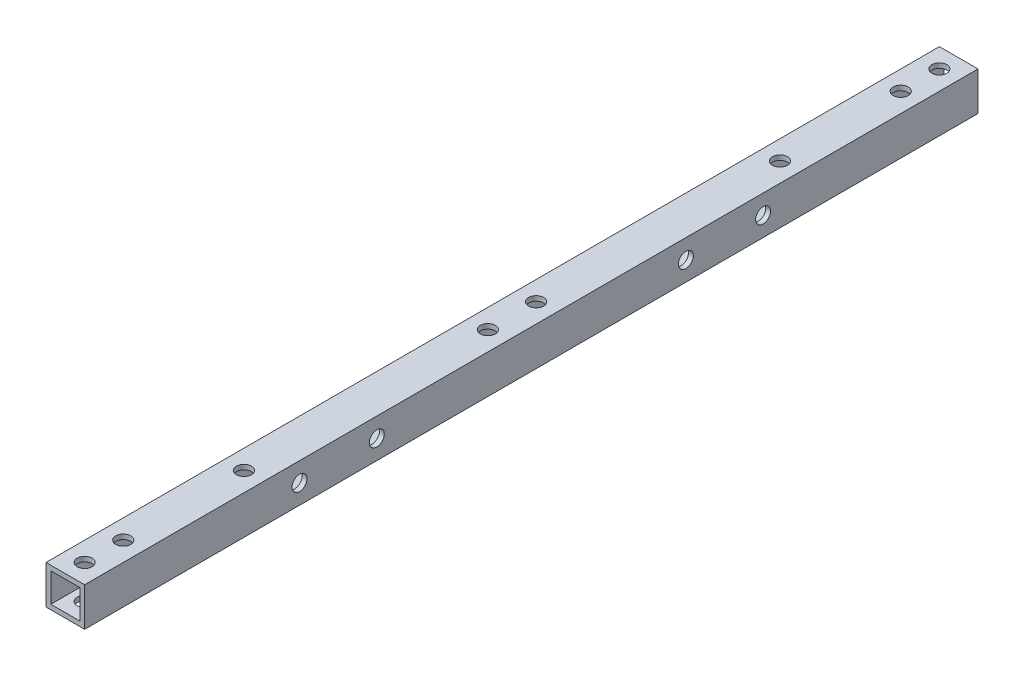
from build123d import *

# Parameters (mm, degrees)
SKETCH_1_W          = 8
SKETCH_1_H          = 8
SKETCH_1_W_2        = 6
SKETCH_1_H_2        = 6
EXTRUDE_1_DEPTH     = 185
SKETCH_2_R          = 1.55
CUT_EXTRUDE_1_DEPTH = 186.216090014
SKETCH_3_R          = 1.55
CUT_EXTRUDE_2_DEPTH = 186.216090014


with BuildPart() as part:
    # 草图1 → 凸台-拉伸1 (new body)
    with BuildSketch(Plane.XY):
        Rectangle(SKETCH_1_W, SKETCH_1_H)
        Rectangle(SKETCH_1_W_2, SKETCH_1_H_2, mode=Mode.SUBTRACT)
    extrude(amount=EXTRUDE_1_DEPTH)

    # 草图2 → 切除-拉伸1 (cut, through all)
    with BuildSketch(Plane(origin=(4, 0, 0), x_dir=(0, 0, -1), z_dir=(1, 0, 0))):
        with Locations(Location((-44.5, 0, 0), (0, 0, 90))):
            Circle(SKETCH_2_R)
        with Locations(Location((-60.5, 0, 0), (0, 0, 90))):
            Circle(SKETCH_2_R)
        with Locations(Location((-124.5, 0, 0), (0, 0, 90))):
            Circle(SKETCH_2_R)
        with Locations(Location((-140.5, 0, 0), (0, 0, 90))):
            Circle(SKETCH_2_R)
    extrude(amount=-CUT_EXTRUDE_1_DEPTH, mode=Mode.SUBTRACT)

    # 草图3 → 切除-拉伸2 (cut, through all)
    with BuildSketch(Plane(origin=(0, 4, 0), x_dir=(1, 0, 0), z_dir=(0, 1, 0))):
        with Locations(Location((0, -4, 0), (0, 0, 270))):
            Circle(SKETCH_3_R)
        with Locations(Location((0, -12, 0), (0, 0, 270))):
            Circle(SKETCH_3_R)
        with Locations(Location((0, -173, 0), (0, 0, 270))):
            Circle(SKETCH_3_R)
        with Locations(Location((0, -181, 0), (0, 0, 270))):
            Circle(SKETCH_3_R)
        with Locations(Location((0, -87.5, 0), (0, 0, 270))):
            Circle(SKETCH_3_R)
        with Locations(Location((0, -97.5, 0), (0, 0, 270))):
            Circle(SKETCH_3_R)
        with Locations(Location((0, -148, 0), (0, 0, 270))):
            Circle(SKETCH_3_R)
        with Locations(Location((0, -37, 0), (0, 0, 270))):
            Circle(SKETCH_3_R)
    extrude(amount=-CUT_EXTRUDE_2_DEPTH, mode=Mode.SUBTRACT)


solid = part.part
